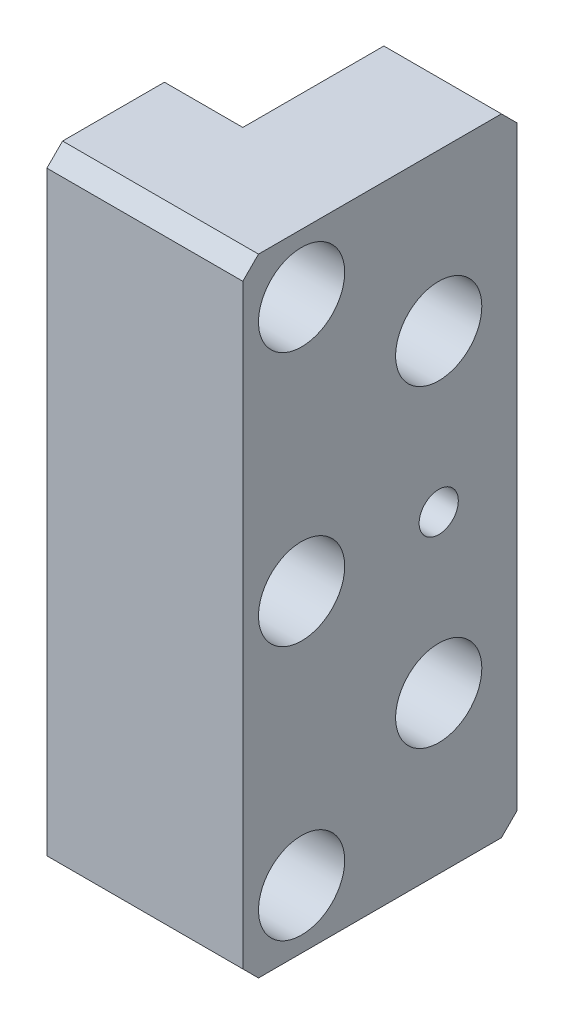
SolidWorks part; units mm, degrees
material "S45C"
ref_plane "前视基准面" through (0, 0, 0) normal (0, 0, 1) x (1, 0, 0)
ref_plane "上视基准面" through (0, 0, 0) normal (0, 1, 0) x (1, 0, 0)
ref_plane "右视基准面" through (0, 0, 0) normal (1, 0, 0) x (0, 0, -1)
sketch "草图1" plane through (0, 0, 0) normal (0, 1, 0) x (1, 0, 0)
  line L0 (0, 0) -> (25, 0)
  line L1 (25, 0) -> (25, 35)
  line L2 (25, 35) -> (10, 35)
  line L3 (10, 35) -> (10, 15)
  line L4 (10, 15) -> (0, 15)
  line L5 (0, 15) -> (0, 0)
  dimension "D1" = 15
  dimension "D2" = 10
  dimension "D3" = 15
  dimension "D4" = 20
extrude "凸台-拉伸1" add sketch "草图1" along normal mid plane 80
chamfer "倒角1" distance 2 angle 45 4 edges at (12.5, -40, 0) (17.5, -40, -35) (12.5, 40, 0) (17.5, 40, -35)
sketch "草图2" plane through (25, 0, 0) normal (1, 0, 0) x (0, 0, -1)
  line L0 (0, 0) -> (27.7409, 0) construction
  line L3 (0, 38) -> (0, -38) construction
  point P0 (7.5, 32.5)
  point P2 (7.5, 0)
  point P4 (7.5, -32.5)
  dimension "D1" = 7.5
  dimension "D2" = 65
hole_wizard "M6 六角圆柱头螺钉的柱形沉头孔1" positions "草图2" profile "草图3" counterbore size "M6" standard "GB" end condition up to next
sketch "草图3" plane through (25, 32.5, -7.5) normal (0, 1, 0) x (0, 0, -1)
  line L0 (0, 0) -> (0, 25)
  line L1 (0, 25) -> (3.3, 25)
  line L3 (3.3, 25) -> (3.3, 15)
  line L4 (3.3, 15) -> (5.5, 15)
  line L5 (5.5, 15) -> (5.5, 0)
  line L7 (5.5, 0) -> (0, 0)
  line L11 (0, -6.35) -> (0, 107.95) construction
  dimension "通孔孔直径" = 6.6
  dimension "通孔孔深度" = 25
  dimension "柱形沉头孔直径" = 11
  dimension "柱形沉头孔深度" = 15
sketch "草图4" plane through (25, 0, 0) normal (1, 0, 0) x (0, 0, -1)
  line L0 (35, 38) -> (35, -38) construction
  point P0 (25, 0)
  dimension "D1" = 10
hole_wizard "M6 螺纹孔1" positions "草图4" profile "草图5" tap size "M6" standard "GB" end condition up to next
sketch "草图5" plane through (25, 0, -25) normal (0, 1, 0) x (0, 0, -1)
  line L0 (0, 0) -> (0, 15)
  line L1 (0, 15) -> (2.5, 15)
  line L2 (2.5, 15) -> (2.5, 0)
  line L5 (2.5, 0) -> (0, 0)
  line L11 (0, -6.35) -> (0, 107.95) construction
  dimension "通孔螺纹孔钻头直径" = 5
  dimension "通孔螺纹孔钻头深度" = 15
cosmetic thread "孔螺纹线1" parameters "D2"=6
sketch "草图6" plane through (25, 0, 0) normal (1, 0, 0) x (0, 0, -1)
  line L0 (0, 0) -> (37.7517, 0) construction
  line L3 (35, 38) -> (35, -38) construction
  point P0 (25, 20)
  point P2 (25, -20)
  dimension "D1" = 10
  dimension "D2" = 40
hole_wizard "M6 六角圆柱头螺钉的柱形沉头孔2" positions "草图6" profile "草图7" counterbore size "M6" standard "GB" end condition up to next
sketch "草图7" plane through (25, 20, -25) normal (0, 1, 0) x (0, 0, -1)
  line L0 (0, 0) -> (0, 15)
  line L1 (0, 15) -> (3.3, 15)
  line L3 (3.3, 15) -> (3.3, 8)
  line L4 (3.3, 8) -> (5.5, 8)
  line L5 (5.5, 8) -> (5.5, 0)
  line L7 (5.5, 0) -> (0, 0)
  line L11 (0, -6.35) -> (0, 107.95) construction
  dimension "通孔孔直径" = 6.6
  dimension "通孔孔深度" = 15
  dimension "柱形沉头孔直径" = 11
  dimension "柱形沉头孔深度" = 8
